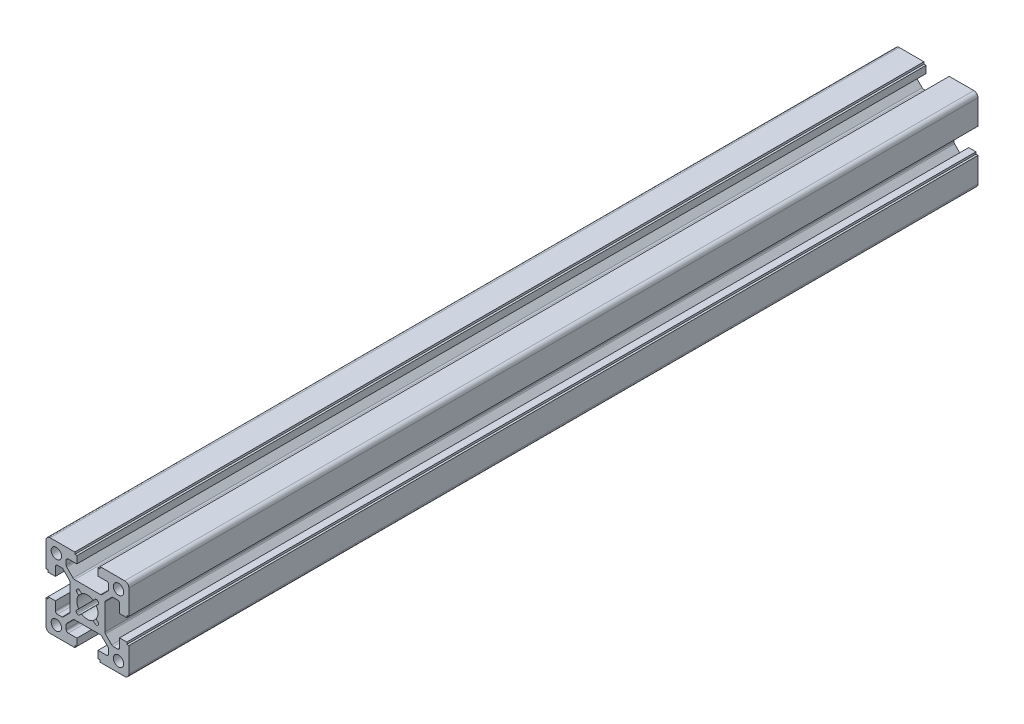
SolidWorks part; units mm, degrees
ref_plane "Front Plane" through (0, 0, 0) normal (0, 0, 1) x (1, 0, 0)
ref_plane "Top Plane" through (0, 0, 0) normal (0, 1, 0) x (1, 0, 0)
ref_plane "Right Plane" through (0, 0, 0) normal (1, 0, 0) x (0, 0, -1)
sketch "Sketch1" plane through (0, 0, 0) normal (0, 0, 1) x (1, 0, 0)
  line L0 (-5.1792, 3.7656) -> (-4.2435, 2.8299)
  line L1 (-4.2435, -2.8281) -> (-5.2772, -3.8618)
  line L2 (-5.2772, -4.9224) -> (-4.924, -5.2756)
  line L3 (-3.8637, -5.276) -> (-2.8295, -4.2431)
  line L4 (2.8295, -4.2431) -> (3.7786, -5.1922)
  line L5 (4.8389, -5.1925) -> (5.193, -4.8389)
  line L6 (5.1933, -3.7779) -> (4.2435, -2.8281)
  line L7 (4.2435, 2.8299) -> (5.1933, 3.7797)
  line L8 (5.1933, 4.8403) -> (4.8393, 5.1943)
  line L9 (3.7783, 5.1939) -> (2.8295, 4.2439)
  line L10 (-2.8295, 4.2439) -> (-3.7652, 5.1796)
  line L11 (-4.8258, 5.1796) -> (-5.1792, 4.8262)
  line L12 (-5.1005, 15.5009) -> (-5.1005, 19.0009)
  line L13 (-9.2505, 15.5009) -> (-5.1005, 15.5009)
  line L14 (-10.2505, 12.4331) -> (-10.2505, 14.5009)
  line L15 (-6.9254, 8.6938) -> (-9.9576, 11.726)
  line L16 (6.2183, 8.4009) -> (-6.2183, 8.4009)
  line L17 (9.9566, 11.725) -> (6.9254, 8.6938)
  line L18 (10.2495, 14.5009) -> (10.2495, 12.4321)
  line L19 (5.0995, 15.5009) -> (9.2495, 15.5009)
  line L20 (5.0995, 19.0009) -> (5.0995, 15.5009)
  line L21 (6.0995, 19.0009) -> (5.0995, 19.0009)
  line L22 (6.0995, 20.0009) -> (6.0995, 19.0009)
  line L23 (17.9995, 20.0009) -> (6.0995, 20.0009)
  line L24 (19.9995, 6.1009) -> (19.9995, 18.0009)
  line L25 (18.9995, 6.1009) -> (19.9995, 6.1009)
  line L26 (18.9995, 5.1009) -> (18.9995, 6.1009)
  line L27 (15.4995, 5.1009) -> (18.9995, 5.1009)
  line L28 (15.4995, 9.2509) -> (15.4995, 5.1009)
  line L29 (12.4317, 10.2509) -> (14.4995, 10.2509)
  line L30 (8.6924, 6.9258) -> (11.7246, 9.958)
  line L31 (8.3995, -6.2169) -> (8.3995, 6.2187)
  line L32 (11.7246, -9.9562) -> (8.6924, -6.924)
  line L33 (14.4995, -10.2491) -> (12.4317, -10.2491)
  line L34 (15.4995, -5.0991) -> (15.4995, -9.2491)
  line L35 (18.9995, -5.0991) -> (15.4995, -5.0991)
  line L36 (18.9995, -6.0991) -> (18.9995, -5.0991)
  line L37 (19.9995, -6.0991) -> (18.9995, -6.0991)
  line L38 (19.9995, -17.9991) -> (19.9995, -6.0991)
  line L39 (6.0995, -19.9991) -> (17.9995, -19.9991)
  line L40 (6.0995, -18.9991) -> (6.0995, -19.9991)
  line L41 (5.0995, -18.9991) -> (6.0995, -18.9991)
  line L42 (5.0995, -15.4991) -> (5.0995, -18.9991)
  line L43 (9.2495, -15.4991) -> (5.0995, -15.4991)
  line L44 (10.2495, -12.4303) -> (10.2495, -14.4991)
  line L45 (6.9254, -8.692) -> (9.9566, -11.7232)
  line L46 (-6.2183, -8.3991) -> (6.2183, -8.3991)
  line L47 (-9.9576, -11.7242) -> (-6.9254, -8.692)
  line L48 (-10.2505, -14.4991) -> (-10.2505, -12.4313)
  line L49 (-5.1005, -15.4991) -> (-9.2505, -15.4991)
  line L50 (-5.1005, -18.9991) -> (-5.1005, -15.4991)
  line L51 (-6.1005, -18.9991) -> (-5.1005, -18.9991)
  line L52 (-6.1005, -19.9991) -> (-6.1005, -18.9991)
  line L53 (-18.0005, -19.9991) -> (-6.1005, -19.9991)
  line L54 (-20.0005, -6.0991) -> (-20.0005, -17.9991)
  line L55 (-19.0005, -6.0991) -> (-20.0005, -6.0991)
  line L56 (-19.0005, -5.0991) -> (-19.0005, -6.0991)
  line L57 (-15.5005, -5.0991) -> (-19.0005, -5.0991)
  line L58 (-15.5005, -9.2491) -> (-15.5005, -5.0991)
  line L59 (-12.4317, -10.2491) -> (-14.5005, -10.2491)
  line L60 (-8.6934, -6.925) -> (-11.7246, -9.9562)
  line L61 (-8.4005, 6.2197) -> (-8.4005, -6.2179)
  line L62 (-11.7246, 9.958) -> (-8.6934, 6.9268)
  line L63 (-14.5005, 10.2509) -> (-12.4317, 10.2509)
  line L64 (-15.5005, 5.1009) -> (-15.5005, 9.2509)
  line L65 (-19.0005, 5.1009) -> (-15.5005, 5.1009)
  line L66 (-19.0005, 6.1009) -> (-19.0005, 5.1009)
  line L67 (-20.0005, 6.1009) -> (-19.0005, 6.1009)
  line L68 (-20.0005, 18.0009) -> (-20.0005, 6.1009)
  line L69 (-6.1005, 20.0009) -> (-18.0005, 20.0009)
  line L70 (-6.1005, 19.0009) -> (-6.1005, 20.0009)
  line L71 (-5.1005, 19.0009) -> (-6.1005, 19.0009)
  arc A0 (-5.1792, 4.8262) -> (-5.1792, 3.7656) centre (-4.6488, 4.2959) ccw
  arc A1 (-4.2435, 2.8299) -> (-4.2435, -2.8281) centre (-0.0001, 0.0009) ccw
  arc A2 (-5.2772, -3.8618) -> (-5.2772, -4.9224) centre (-4.7468, -4.3921) ccw
  arc A3 (-4.924, -5.2756) -> (-3.8637, -5.276) centre (-4.3937, -4.7453) ccw
  arc A4 (-2.8295, -4.2431) -> (2.8295, -4.2431) centre (0, 0) ccw
  arc A5 (3.7786, -5.1922) -> (4.8389, -5.1925) centre (4.3089, -4.6619) ccw
  arc A6 (5.193, -4.8389) -> (5.1933, -3.7779) centre (4.663, -4.3083) ccw
  arc A7 (4.2435, -2.8281) -> (4.2435, 2.8299) centre (0.0001, 0.0009) ccw
  arc A8 (5.1933, 3.7797) -> (5.1933, 4.8403) centre (4.6629, 4.31) ccw
  arc A9 (4.8393, 5.1943) -> (3.7783, 5.1939) centre (4.309, 4.6639) ccw
  arc A10 (2.8295, 4.2439) -> (-2.8295, 4.2439) centre (0, 0.0008) ccw
  arc A11 (-3.7652, 5.1796) -> (-4.8258, 5.1796) centre (-4.2955, 4.6492) ccw
  circle A12 centre (-15.0005, 15.0009) radius 2.5
  circle A13 centre (14.9995, -14.9991) radius 2.5
  arc A14 (-9.2505, 15.5009) -> (-10.2505, 14.5009) centre (-9.2505, 14.5009) ccw
  arc A15 (-10.2505, 12.4331) -> (-9.9576, 11.726) centre (-9.2505, 12.4331) ccw
  arc A16 (-6.9254, 8.6938) -> (-6.2183, 8.4009) centre (-6.2183, 9.4009) ccw
  arc A17 (6.2183, 8.4009) -> (6.9254, 8.6938) centre (6.2183, 9.4009) ccw
  arc A18 (9.9566, 11.725) -> (10.2495, 12.4321) centre (9.2495, 12.4321) ccw
  arc A19 (10.2495, 14.5009) -> (9.2495, 15.5009) centre (9.2495, 14.5009) ccw
  arc A20 (19.9995, 18.0009) -> (17.9995, 20.0009) centre (17.9995, 18.0009) ccw
  arc A21 (15.4995, 9.2509) -> (14.4995, 10.2509) centre (14.4995, 9.2509) ccw
  arc A22 (12.4317, 10.2509) -> (11.7246, 9.958) centre (12.4317, 9.2509) ccw
  arc A23 (8.6924, 6.9258) -> (8.3995, 6.2187) centre (9.3995, 6.2187) ccw
  arc A24 (8.3995, -6.2169) -> (8.6924, -6.924) centre (9.3995, -6.2169) ccw
  arc A25 (11.7246, -9.9562) -> (12.4317, -10.2491) centre (12.4317, -9.2491) ccw
  arc A26 (14.4995, -10.2491) -> (15.4995, -9.2491) centre (14.4995, -9.2491) ccw
  arc A27 (17.9995, -19.9991) -> (19.9995, -17.9991) centre (17.9995, -17.9991) ccw
  arc A28 (9.2495, -15.4991) -> (10.2495, -14.4991) centre (9.2495, -14.4991) ccw
  arc A29 (10.2495, -12.4303) -> (9.9566, -11.7232) centre (9.2495, -12.4303) ccw
  arc A30 (6.9254, -8.692) -> (6.2183, -8.3991) centre (6.2183, -9.3991) ccw
  arc A31 (-6.2183, -8.3991) -> (-6.9254, -8.692) centre (-6.2183, -9.3991) ccw
  arc A32 (-9.9576, -11.7242) -> (-10.2505, -12.4313) centre (-9.2505, -12.4313) ccw
  arc A33 (-10.2505, -14.4991) -> (-9.2505, -15.4991) centre (-9.2505, -14.4991) ccw
  arc A34 (-20.0005, -17.9991) -> (-18.0005, -19.9991) centre (-18.0005, -17.9991) ccw
  arc A35 (-15.5005, -9.2491) -> (-14.5005, -10.2491) centre (-14.5005, -9.2491) ccw
  arc A36 (-12.4317, -10.2491) -> (-11.7246, -9.9562) centre (-12.4317, -9.2491) ccw
  arc A37 (-8.6934, -6.925) -> (-8.4005, -6.2179) centre (-9.4005, -6.2179) ccw
  arc A38 (-8.4005, 6.2197) -> (-8.6934, 6.9268) centre (-9.4005, 6.2197) ccw
  arc A39 (-11.7246, 9.958) -> (-12.4317, 10.2509) centre (-12.4317, 9.2509) ccw
  arc A40 (-14.5005, 10.2509) -> (-15.5005, 9.2509) centre (-14.5005, 9.2509) ccw
  arc A41 (-18.0005, 20.0009) -> (-20.0005, 18.0009) centre (-18.0005, 18.0009) ccw
  circle A42 centre (-15.0005, -14.9991) radius 2.5
  circle A43 centre (14.9995, 15.0009) radius 2.5
extrude "Boss-Extrude1" add sketch "Sketch1" along normal mid plane 410
